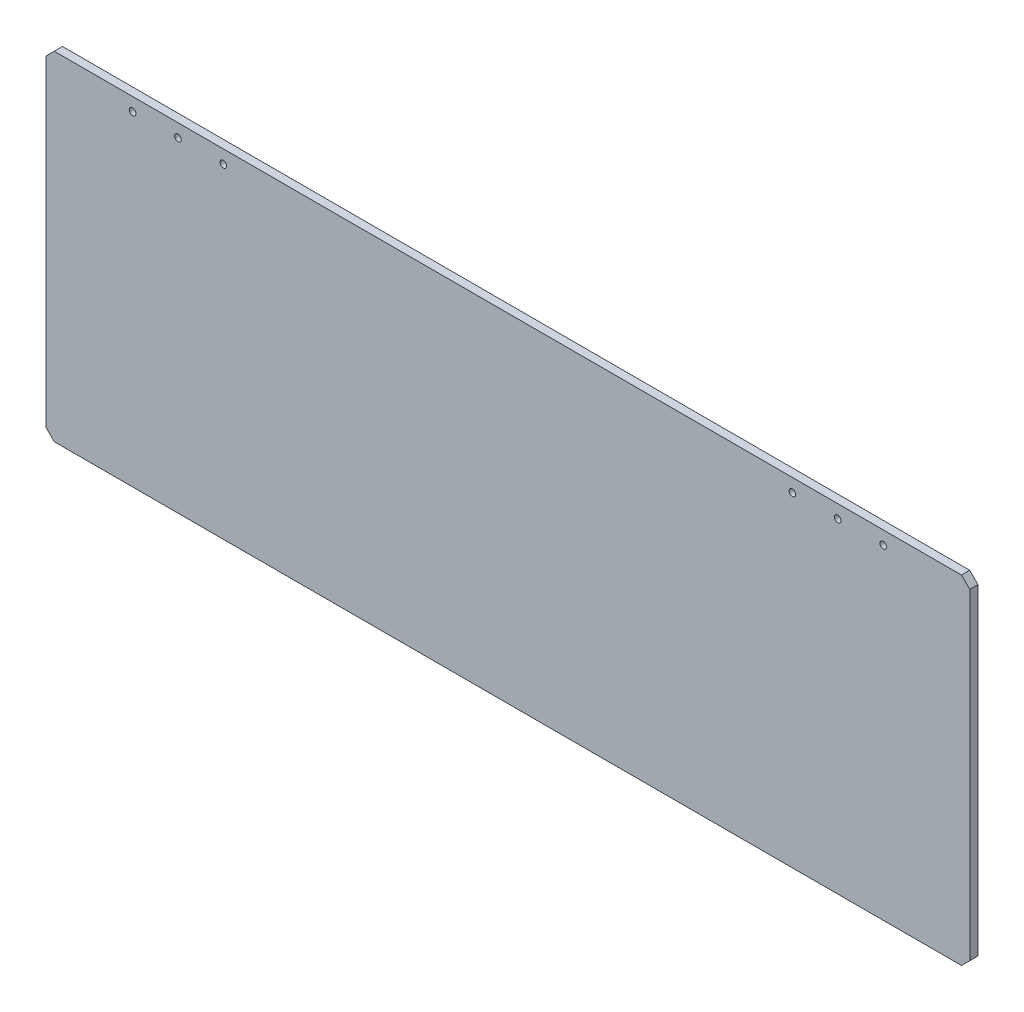
SolidWorks part; units mm, degrees
material "普通碳钢"
ref_plane "Front Plane" through (0, 0, 0) normal (0, 0, 1) x (1, 0, 0)
ref_plane "Top Plane" through (0, 0, 0) normal (0, 1, 0) x (1, 0, 0)
ref_plane "Right Plane" through (0, 0, 0) normal (1, 0, 0) x (0, 0, -1)
sketch "Sketch1" plane through (0, 0, 0) normal (0, 0, 1) x (1, 0, 0)
  line L0 (0, -5) -> (5, 0)
  line L1 (5, 0) -> (555, 0)
  line L2 (0, -5) -> (0, -200)
  line L3 (5, -205) -> (555, -205)
  line L4 (560, -5) -> (560, -200)
  line L5 (0, 0) -> (560, -205) construction
  line L6 (0, -205) -> (560, 0) construction
  line L7 (555, 0) -> (560, -5)
  line L8 (560, -200) -> (555, -205)
  line L9 (0, -200) -> (5, -205)
  line L10 (280, 0) -> (280, -200) construction
  circle A0 centre (52.5, -8) radius 2
  circle A1 centre (80, -8) radius 2
  circle A2 centre (107.5, -8) radius 2
  circle A3 centre (452.5, -8) radius 2
  circle A4 centre (480, -8) radius 2
  circle A5 centre (507.5, -8) radius 2
  point P4 (280, -102.5)
  dimension "D10" = 4
  dimension "D1" = 560
  dimension "D2" = 205
  dimension "D3" = 27.5
  dimension "D4" = 27.5
  dimension "D5" = 8
  dimension "D11" = 400
extrude "Boss-Extrude1" add sketch "Sketch1" along normal blind 5
cosmetic thread "Cosmetic Thread2" parameters "D2"=5
cosmetic thread "Cosmetic Thread3" parameters "D2"=5
cosmetic thread "Cosmetic Thread4" parameters "D2"=5
